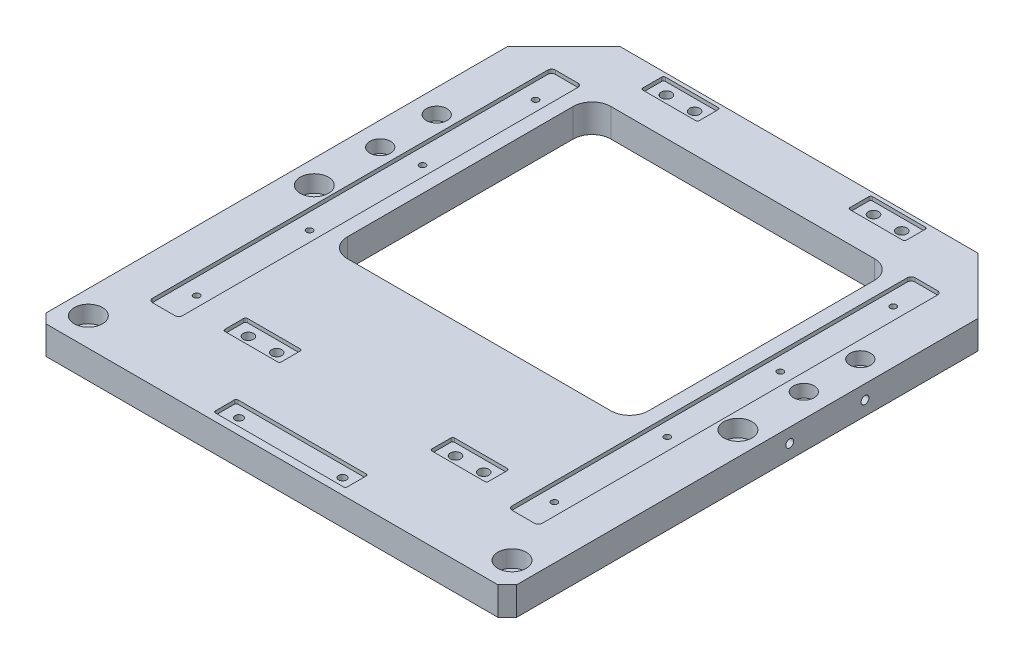
SolidWorks part; units mm, degrees
material "45#"
ref_plane "前基準面" through (0, 0, 0) normal (0, 0, 1) x (1, 0, 0)
ref_plane "上基準面" through (0, 0, 0) normal (0, 1, 0) x (1, 0, 0)
ref_plane "右基準面" through (0, 0, 0) normal (1, 0, 0) x (0, 0, -1)
sketch "草图1" plane through (0, 0, 0) normal (0, 1, 0) x (1, 0, 0)
  line L1 (-125, -140) -> (125, -140)
  line L2 (-125, -140) -> (-125, 140)
  line L3 (-125, 140) -> (125, 140)
  line L4 (125, -140) -> (125, 140)
  line L5 (-125, -140) -> (125, 140) construction
  line L6 (-125, 140) -> (125, -140) construction
  point P0 (0, 0)
  dimension "D1" = 250
  dimension "D2" = 280
extrude "凸台-拉伸1" add sketch "草图1" along normal mid plane 15
sketch "草图2" plane through (0, 7.5, 0) normal (0, 1, 0) x (1, 0, 0)
  line L0 (0, 0) -> (0, -108.98) construction
  line L2 (-125, 140) -> (-125, -140) construction
  line L5 (-125, -140) -> (125, -140) construction
  point P0 (-112.5, -125)
  point P17 (112.5, -125)
  point P18 (112.5, -5)
  point P20 (-112.5, -5)
  dimension "D3" = 12.5
  dimension "D4" = 15
  dimension "D5" = 120
  dimension "D1" = 2
  dimension "D2" = 2
hole_wizard "M8 六角圆柱头螺钉的柱形沉头孔2" positions "草图2" profile "草图3" counterbore size "M8" standard "GB" end condition through all
sketch "草图3" plane through (-112.5, 7.5, 125) normal (1, 0, 0) x (0, 0, 1)
  line L0 (0, 0) -> (0, 15)
  line L1 (0, 15) -> (4.5, 15)
  line L3 (4.5, 15) -> (4.5, 9)
  line L4 (4.5, 9) -> (7.5, 9)
  line L5 (7.5, 9) -> (7.5, 0)
  line L7 (7.5, 0) -> (0, 0)
  line L11 (0, -6.35) -> (0, 107.95) construction
  dimension "通孔孔直径" = 9
  dimension "通孔孔深度" = 15
  dimension "柱形沉头孔直径" = 15
  dimension "柱形沉头孔深度" = 9
sketch "草图4" plane through (0, 7.5, 0) normal (0, 1, 0) x (1, 0, 0)
  line L0 (0, -30) -> (0, -140) construction
  line L1 (-70, -30) -> (70, -30)
  line L2 (-80, -20) -> (-80, 100)
  line L3 (-70, 110) -> (70, 110)
  line L4 (80, -20) -> (80, 100)
  line L5 (-125, -140) -> (125, -140) construction
  line L6 (125, 140) -> (-125, 140) construction
  arc A0 (-80, 100) -> (-70, 110) centre (-70, 100) cw
  arc A1 (80, 100) -> (70, 110) centre (70, 100) ccw
  arc A2 (70, -30) -> (80, -20) centre (70, -20) ccw
  arc A3 (-80, -20) -> (-70, -30) centre (-70, -20) ccw
  dimension "D1" = 10
  dimension "D2" = 30
  dimension "D3" = 160
  dimension "D4" = 140
extrude "切除-拉伸1" cut sketch "草图4" against normal up to surface (15 mm away) up to face at (-112.5, -7.5, 129.5)
sketch "草图5" plane through (0, 7.5, 0) normal (0, 1, 0) x (1, 0, 0)
  line L0 (0, 195.533) -> (0, 0) construction
  line L2 (125, 140) -> (-125, 140) construction
  point P0 (95, 95)
  point P9 (-95, 95)
  point P10 (-95, 35)
  point P11 (-95, -25)
  point P12 (-95, -85)
  point P13 (95, 35)
  point P14 (95, -25)
  point P15 (95, -85)
  dimension "D3" = 190
  dimension "D4" = 45
  dimension "D5" = 60
  dimension "D1" = 2
  dimension "D2" = 4
hole_wizard "M4 螺纹孔1" positions "草图5" profile "草图6" tap size "M4" standard "GB" end condition through all
sketch "草图6" plane through (95, 7.5, -95) normal (1, 0, 0) x (0, 0, 1)
  line L0 (0, 0) -> (0, 15)
  line L1 (0, 15) -> (1.65, 15)
  line L2 (1.65, 15) -> (1.65, 0)
  line L5 (1.65, 0) -> (0, 0)
  line L11 (0, -6.35) -> (0, 107.95) construction
  dimension "通孔螺纹孔钻头直径" = 3.3
  dimension "通孔螺纹孔钻头深度" = 15
cosmetic thread "孔螺纹线27" parameters "D2"=4
cosmetic thread "孔螺纹线28" parameters "D2"=4
cosmetic thread "孔螺纹线29" parameters "D2"=4
cosmetic thread "孔螺纹线30" parameters "D2"=4
cosmetic thread "孔螺纹线31" parameters "D2"=4
cosmetic thread "孔螺纹线32" parameters "D2"=4
cosmetic thread "孔螺纹线33" parameters "D2"=4
cosmetic thread "孔螺纹线34" parameters "D2"=4
sketch "草图7" plane through (0, 7.5, 0) normal (0, 1, 0) x (1, 0, 0)
  line L0 (0, 0) -> (0, -130.212) construction
  line L2 (-125, -140) -> (125, -140) construction
  point P0 (27.5, -130)
  point P9 (-27.5, -130)
  dimension "D1" = 55
  dimension "D2" = 10
hole_wizard "M5 螺纹孔1" positions "草图7" profile "草图8" tap size "M5" standard "GB" end condition through all
sketch "草图8" plane through (27.5, 7.5, 130) normal (1, 0, 0) x (0, 0, 1)
  line L0 (0, 0) -> (0, 15)
  line L1 (0, 15) -> (2.1, 15)
  line L2 (2.1, 15) -> (2.1, 0)
  line L5 (2.1, 0) -> (0, 0)
  line L11 (0, -6.35) -> (0, 107.95) construction
  dimension "通孔螺纹孔钻头直径" = 4.2
  dimension "通孔螺纹孔钻头深度" = 15
cosmetic thread "孔螺纹线11" parameters "D2"=5
cosmetic thread "孔螺纹线12" parameters "D2"=5
sketch "草图9" plane through (0, -7.5, 0) normal (0, -1, 0) x (-1, 0, 0)
  line L0 (55, 107.5) -> (55, 129.1956) construction
  line L5 (95, 21) -> (-43.0463, 21) construction
  line L7 (0, 196.5472) -> (0, 0) construction
  line L8 (-125, 140) -> (125, 140) construction
  line L9 (125, -140) -> (-125, -140) construction
  point P0 (47.5, 132)
  point P19 (62.5, 132)
  point P20 (62.5, -90)
  point P21 (47.5, -90)
  point P27 (-47.5, -90)
  point P28 (-62.5, -90)
  point P29 (-62.5, 132)
  point P30 (-47.5, 132)
  dimension "D1" = 15
  dimension "D2" = 8
  dimension "D3" = 55
  dimension "D4" = 50
hole_wizard "M5 六角圆柱头螺钉的柱形沉头孔2" positions "草图9" profile "草图10" counterbore size "M5" standard "GB" end condition through all
sketch "草图10" plane through (-47.5, -7.5, -132) normal (1, 0, 0) x (0, 0, -1)
  line L0 (0, 0) -> (0, 15)
  line L1 (0, 15) -> (2.75, 15)
  line L3 (2.75, 15) -> (2.75, 5.7)
  line L4 (2.75, 5.7) -> (5, 5.7)
  line L5 (5, 5.7) -> (5, 0)
  line L7 (5, 0) -> (0, 0)
  line L11 (0, -6.35) -> (0, 107.95) construction
  dimension "通孔孔直径" = 5.5
  dimension "通孔孔深度" = 15
  dimension "柱形沉头孔直径" = 10
  dimension "柱形沉头孔深度" = 5.7
sketch "草图11" plane through (0, 7.5, 0) normal (0, 1, 0) x (1, 0, 0)
  line L0 (0, 0) -> (0, 170.999) construction
  line L1 (101.5, -102) -> (89.5, -102)
  line L2 (103.5, -100) -> (103.5, 110)
  line L3 (101.5, 112) -> (89.5, 112)
  line L4 (87.5, -100) -> (87.5, 110)
  line L5 (-87.5, -100) -> (-87.5, 110)
  line L6 (-101.5, 112) -> (-89.5, 112)
  line L7 (-103.5, -100) -> (-103.5, 110)
  line L8 (-101.5, -102) -> (-89.5, -102)
  circle A0 centre (95, -85) radius 1.65 construction
  circle A1 centre (95, 95) radius 1.65 construction
  arc A2 (89.5, 112) -> (87.5, 110) centre (89.5, 110) ccw
  arc A3 (103.5, 110) -> (101.5, 112) centre (101.5, 110) ccw
  arc A4 (89.5, -102) -> (87.5, -100) centre (89.5, -100) cw
  arc A5 (101.5, -102) -> (103.5, -100) centre (101.5, -100) ccw
  arc A6 (-101.5, -102) -> (-103.5, -100) centre (-101.5, -100) cw
  arc A7 (-89.5, -102) -> (-87.5, -100) centre (-89.5, -100) ccw
  arc A8 (-103.5, 110) -> (-101.5, 112) centre (-101.5, 110) cw
  arc A9 (-89.5, 112) -> (-87.5, 110) centre (-89.5, 110) cw
  point P14 (87.5, -102)
  point P17 (103.5, -102)
extrude "切除-拉伸2" cut sketch "草图11" against normal blind 2
hole_wizard "M6 六角圆柱头螺钉的柱形沉头孔1" positions "草图12" profile "草图13" counterbore size "M6" standard "GB"
sketch "草图12" plane through (0, 7.5, 0) normal (0, 1, 0) x (1, 0, 0)
  line L1 (-112.5, -5) -> (-112.5, 162.0109) construction
  line L3 (0, 0) -> (0, 188.8808) construction
  circle A0 centre (-112.5, -5) radius 7.5 construction
  point P0 (-112.5, 30)
  point P2 (-112.5, 60)
  point P21 (112.5, 60)
  point P22 (112.5, 30)
  dimension "D1" = 35
  dimension "D2" = 30
sketch "草图13" plane through (-112.5, 7.5, -30) normal (1, 0, 0) x (0, 0, 1)
  line L0 (0, 0) -> (0, 16.9828)
  line L1 (0, 16.9828) -> (3.3, 15)
  line L2 (3.3, 15) -> (3.3, 6.8)
  line L3 (3.3, 6.8) -> (5.5, 6.8)
  line L4 (5.5, 6.8) -> (5.5, 0)
  line L5 (5.5, 0) -> (0, 0)
  line L10 (0, 16.9828) -> (-3.3, 15) construction
  line L11 (0, -6.35) -> (0, 107.95) construction
  dimension "孔直径" = 6.6
  dimension "孔深度" = 15
  dimension "柱形沉头孔直径" = 11
  dimension "柱形沉头孔深度" = 6.8
  dimension "导头角度" = 118
sketch "草图14" plane through (0, 7.5, 0) normal (0, 1, 0) x (1, 0, 0)
  line L0 (-47.5, 132) -> (-77.3878, 132) construction
  line L1 (-41, 138) -> (-69, 138)
  line L2 (-40, 137) -> (-40, 127)
  line L3 (-41, 126) -> (-69, 126)
  line L4 (-70, 137) -> (-70, 127)
  line L5 (-55, 138) -> (-55, 146.7727) construction
  line L6 (0, 0) -> (0, 197.6716) construction
  line L7 (55, 138) -> (55, 146.7727) construction
  line L8 (47.5, 132) -> (77.3878, 132) construction
  line L9 (70, 137) -> (70, 127)
  line L10 (41, 126) -> (69, 126)
  line L11 (40, 137) -> (40, 127)
  line L12 (41, 138) -> (69, 138)
  line L13 (0, 21) -> (-231.4482, 21) construction
  line L14 (47.5, -90) -> (77.3878, -90) construction
  line L15 (55, -96) -> (55, -104.7727) construction
  line L16 (-55, -96) -> (-55, -104.7727) construction
  line L17 (-47.5, -90) -> (-77.3878, -90) construction
  line L18 (41, -96) -> (69, -96)
  line L19 (40, -95) -> (40, -85)
  line L20 (41, -84) -> (69, -84)
  line L21 (70, -95) -> (70, -85)
  line L22 (-70, -95) -> (-70, -85)
  line L23 (-41, -84) -> (-69, -84)
  line L24 (-40, -95) -> (-40, -85)
  line L25 (-41, -96) -> (-69, -96)
  arc A0 (-69, 126) -> (-70, 127) centre (-69, 127) cw
  arc A1 (-69, 138) -> (-70, 137) centre (-69, 137) ccw
  arc A2 (-41, 138) -> (-40, 137) centre (-41, 137) cw
  arc A3 (-40, 127) -> (-41, 126) centre (-41, 127) cw
  circle A4 centre (-47.5, 132) radius 2.75 construction
  circle A5 centre (-62.5, 132) radius 2.75 construction
  arc A6 (40, 127) -> (41, 126) centre (41, 127) ccw
  arc A7 (41, 138) -> (40, 137) centre (41, 137) ccw
  arc A8 (69, 138) -> (70, 137) centre (69, 137) cw
  arc A9 (69, 126) -> (70, 127) centre (69, 127) ccw
  circle A10 centre (47.5, -90) radius 2.75 construction
  circle A11 centre (47.5, 132) radius 2.75 construction
  arc A12 (69, -84) -> (70, -85) centre (69, -85) cw
  arc A13 (69, -96) -> (70, -95) centre (69, -95) ccw
  arc A14 (41, -96) -> (40, -95) centre (41, -95) cw
  arc A15 (40, -85) -> (41, -84) centre (41, -85) cw
  arc A16 (-40, -85) -> (-41, -84) centre (-41, -85) ccw
  arc A17 (-41, -96) -> (-40, -95) centre (-41, -95) ccw
  arc A18 (-69, -96) -> (-70, -95) centre (-69, -95) cw
  arc A19 (-69, -84) -> (-70, -85) centre (-69, -85) ccw
  point P8 (-70, 138)
  point P11 (-40, 138)
  point P14 (-40, 126)
  point P43 (40, 126)
  point P44 (40, 138)
  point P45 (70, 138)
  point P85 (70, -96)
  point P86 (40, -96)
  point P87 (40, -84)
  point P88 (-40, -84)
  point P89 (-40, -96)
  point P90 (-70, -96)
  dimension "D3" = 1
  dimension "D1" = 12
  dimension "D2" = 30
extrude "切除-拉伸3" cut sketch "草图14" against normal blind 2
sketch "草图15" plane through (0, 7.5, 0) normal (0, 1, 0) x (1, 0, 0)
  line L0 (0, -124) -> (0, -169.8725) construction
  line L1 (34, -124) -> (-34, -124)
  line L2 (35, -125) -> (35, -135)
  line L3 (34, -136) -> (-34, -136)
  line L4 (-35, -125) -> (-35, -135)
  line L5 (27.5, -130) -> (-36.4587, -130) construction
  arc A0 (-34, -136) -> (-35, -135) centre (-34, -135) cw
  arc A1 (-34, -124) -> (-35, -125) centre (-34, -125) ccw
  arc A2 (34, -124) -> (35, -125) centre (34, -125) cw
  arc A3 (35, -135) -> (34, -136) centre (34, -135) cw
  circle A4 centre (27.5, -130) radius 2.1 construction
  circle A5 centre (-27.5, -130) radius 2.1 construction
  point P8 (-35, -124)
  point P11 (35, -124)
  point P14 (35, -136)
  dimension "D3" = 1
  dimension "D1" = 12
  dimension "D2" = 70
extrude "切除-拉伸4" cut sketch "草图15" against normal blind 2
chamfer "倒角1" distance 5 angle 45 2 edges at (-125, 0, 140) (125, 0, 140)
chamfer "倒角2" distance 30 angle 45 2 edges at (125, 0, -140) (-125, 0, -140)
sketch "草图16" plane through (125, 0, 0) normal (1, 0, 0) x (0, 0, -1)
  line L0 (-140, -7.5) -> (-140, 7.5) construction
  point P0 (10, 0)
  point P2 (50, 0)
  dimension "D1" = 40
  dimension "D2" = 150
hole_wizard "M5 螺纹孔2" positions "草图16" profile "草图17" tap size "M5" standard "GB"
sketch "草图17" plane through (125, 0, -10) normal (0, 1, 0) x (0, 0, -1)
  line L0 (0, 0) -> (0, 13.6618)
  line L1 (0, 13.6618) -> (2.1, 12.4)
  line L2 (2.1, 12.4) -> (2.1, 0)
  line L5 (2.1, 0) -> (0, 0)
  line L10 (0, 13.6618) -> (-2.1, 12.4) construction
  line L11 (0, -6.35) -> (0, 107.95) construction
  dimension "螺纹孔钻头直径" = 4.2
  dimension "螺纹孔钻头深度" = 12.4
  dimension "导头角度" = 118
cosmetic thread "孔螺纹线13" parameters "D1"=10, "D2"=5
cosmetic thread "孔螺纹线14" parameters "D1"=10, "D2"=5
equation "\"D4@草图11\"=\"D1@草图11\""
